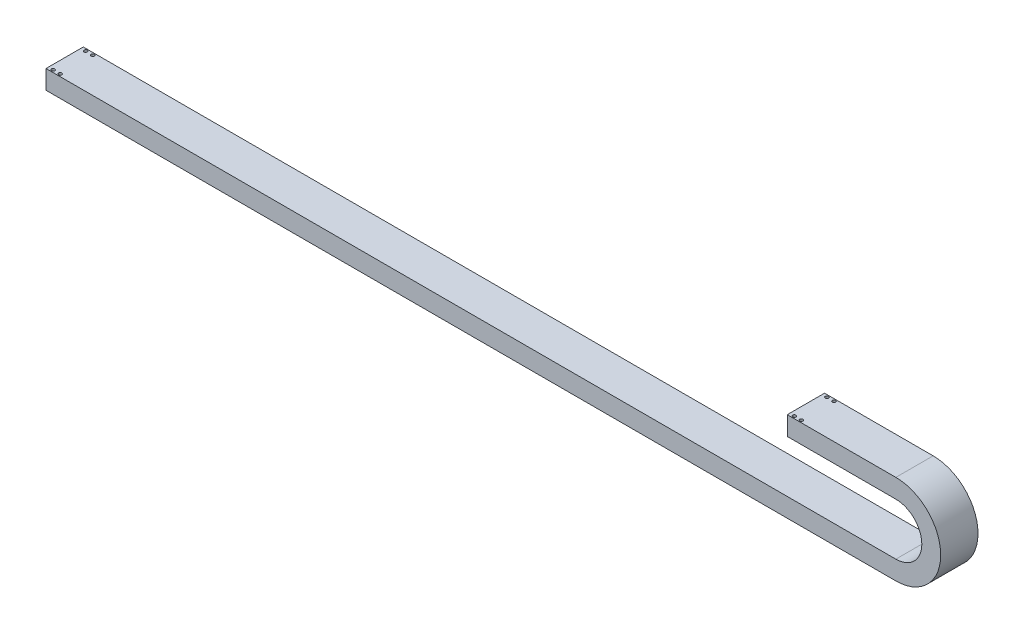
SolidWorks part; units mm, degrees
ref_plane "前视基准面" through (0, 0, 0) normal (0, 0, 1) x (1, 0, 0)
ref_plane "上视基准面" through (0, 0, 0) normal (0, 1, 0) x (1, 0, 0)
ref_plane "右视基准面" through (0, 0, 0) normal (1, 0, 0) x (0, 0, -1)
sketch "草图1" plane through (0, 0, 0) normal (0, 0, 1) x (1, 0, 0)
  line L0 (-327.9007, 39.4094) -> (-97.9007, 39.4094) construction
  line L1 (-327.9007, 19.4094) -> (-97.9007, 19.4094)
  line L2 (-97.9007, -110.5906) -> (-1897.9007, -110.5906) construction
  line L3 (-97.9007, -90.5906) -> (-1897.9007, -90.5906)
  line L4 (-327.9007, 59.4094) -> (-97.9007, 59.4094)
  line L5 (-97.9007, -130.5906) -> (-1897.9007, -130.5906)
  line L6 (-327.9007, 59.4094) -> (-327.9007, 19.4094)
  line L7 (-327.9007, 19.4094) -> (-321.4095, 4.5847)
  line L8 (-1897.9007, -90.5906) -> (-1897.9007, -130.5906)
  line L9 (-1897.9007, -130.5906) -> (-1901.6528, -131.9566)
  arc A0 (-97.9007, -110.5906) -> (-97.9007, 39.4094) centre (-97.9007, -35.5906) ccw construction
  arc A1 (-97.9007, -90.5906) -> (-97.9007, 19.4094) centre (-97.9007, -35.5906) ccw
  arc A2 (-97.9007, -130.5906) -> (-97.9007, 59.4094) centre (-97.9007, -35.5906) ccw
  dimension "D1" = 1800
  dimension "D2" = 150
  dimension "D3" = 230
  dimension "D4" = 20
  dimension "D5" = 20
extrude "凸台-拉伸1" add sketch "草图1" along normal blind 79
hole_wizard "Ø7.0 (7) 直径孔1" positions "草图2" profile "草图3" hole size "Ø7.0" standard "GB" end condition up to next
sketch "草图2" plane through (0, -130.5906, 0) normal (0, -1, 0) x (-1, 0, 0)
  line L0 (1897.9007, -39.5) -> (291.1411, -39.5) construction
  line L1 (1897.9007, -79) -> (1897.9007, 0) construction
  point P0 (1872.9007, -5)
  point P2 (1887.9007, -5)
  point P4 (1872.9007, -74)
  point P6 (1887.9007, -74)
  dimension "D1" = 69
  dimension "D2" = 15
  dimension "D3" = 10
sketch "草图3" plane through (-1872.9007, -130.5906, 5) normal (1, 0, 0) x (0, 0, -1)
  line L0 (0, 0) -> (0, 40)
  line L1 (0, 40) -> (3.5, 40)
  line L2 (3.5, 40) -> (3.5, 0)
  line L5 (3.5, 0) -> (0, 0)
  line L11 (0, -6.35) -> (0, 107.95) construction
  dimension "通孔孔直径" = 7
  dimension "通孔孔深度" = 40
hole_wizard "Ø7.0 (7) 直径孔2" positions "草图4" profile "草图5" hole size "Ø7.0" standard "GB"
sketch "草图4" plane through (0, 59.4094, 0) normal (0, 1, 0) x (1, 0, 0)
  line L0 (-327.9007, -39.5) -> (-316.9054, -39.5) construction
  line L1 (-327.9007, -79) -> (-327.9007, 0) construction
  point P0 (-317.9007, -5)
  point P2 (-302.9007, -5)
  point P4 (-317.9007, -74)
  point P6 (-302.9007, -74)
  dimension "D1" = 69
  dimension "D2" = 15
  dimension "D3" = 10
sketch "草图5" plane through (-317.9007, 59.4094, 5) normal (1, 0, 0) x (0, 0, 1)
  line L0 (0, 0) -> (0, 40)
  line L1 (0, 40) -> (3.5, 40)
  line L2 (3.5, 40) -> (3.5, 0)
  line L5 (3.5, 0) -> (0, 0)
  line L11 (0, -6.35) -> (0, 107.95) construction
  dimension "通孔孔直径" = 7
  dimension "通孔孔深度" = 40
